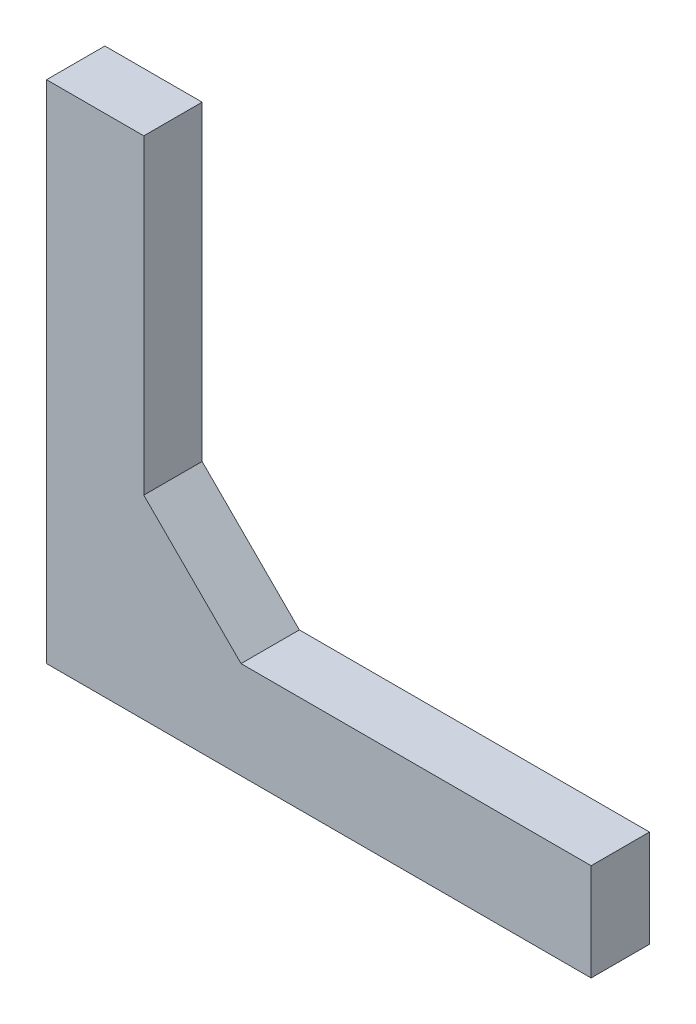
SolidWorks part; units mm, degrees
material "6061 合金"
ref_plane "前视基准面" through (0, 0, 0) normal (0, 0, 1) x (1, 0, 0)
ref_plane "上视基准面" through (0, 0, 0) normal (0, 1, 0) x (1, 0, 0)
ref_plane "右视基准面" through (0, 0, 0) normal (1, 0, 0) x (0, 0, -1)
sketch "草图1" plane through (0, 0, 0) normal (0, 0, 1) x (1, 0, 0)
  line L0 (0, 130) -> (0, 0)
  line L1 (0, 0) -> (140, 0)
  line L2 (140, 0) -> (140, 25)
  line L3 (140, 25) -> (50, 25)
  line L4 (50, 25) -> (25, 50)
  line L5 (25, 50) -> (25, 130)
  line L6 (25, 130) -> (0, 130)
  dimension "D1" = 25
  dimension "D2" = 25
  dimension "D3" = 140
  dimension "D4" = 130
  dimension "D5" = 80
  dimension "D6" = 90
extrude "凸台-拉伸1" add sketch "草图1" along normal mid plane 15
hole_wizard "M6 螺纹孔1" positions "3D草图1" profile "草图2" tap size "M6" standard "GB"
sketch3d "3D草图1"
  line L0 (0, 0, 7.5) -> (140, 0, 7.5) construction
  line L1 (0, 0, 7.5) -> (0, 0, -7.5) construction
  line L2 (0, 130, 7.5) -> (0, 0, 7.5) construction
  point P0 (122.5, 0, 0)
  point P2 (72.5, 0, 0)
  point P4 (22.5, 0, 0)
  point P6 (0, 30, 0)
  point P8 (0, 75, 0)
  point P10 (0, 120, 0)
  dimension "D1" = 7.5
  dimension "D2" = 22.5
  dimension "D3" = 7.5
  dimension "D4" = 7.5
  dimension "D5" = 72.5
  dimension "D6" = 50
  dimension "D7" = 7.5
  dimension "D8" = 7.5
  dimension "D9" = 7.5
  dimension "D10" = 30
  dimension "D11" = 45
  dimension "D12" = 45
sketch "草图2" plane through (122.5, 0, 0) normal (1, 0, 0) x (0, 0, -1)
  line L0 (0, 0) -> (0, 14.0022)
  line L1 (0, 14.0022) -> (2.5, 12.5)
  line L2 (2.5, 12.5) -> (2.5, 0)
  line L5 (2.5, 0) -> (0, 0)
  line L10 (0, 14.0022) -> (-2.5, 12.5) construction
  line L11 (0, -6.35) -> (0, 107.95) construction
  dimension "螺纹孔钻头直径" = 5
  dimension "螺纹孔钻头深度" = 12.5
  dimension "导头角度" = 118
cosmetic thread "孔螺蚊线1"
cosmetic thread "孔螺蚊线2"
cosmetic thread "孔螺蚊线3"
cosmetic thread "孔螺蚊线4"
cosmetic thread "孔螺蚊线5"
cosmetic thread "孔螺蚊线6"
